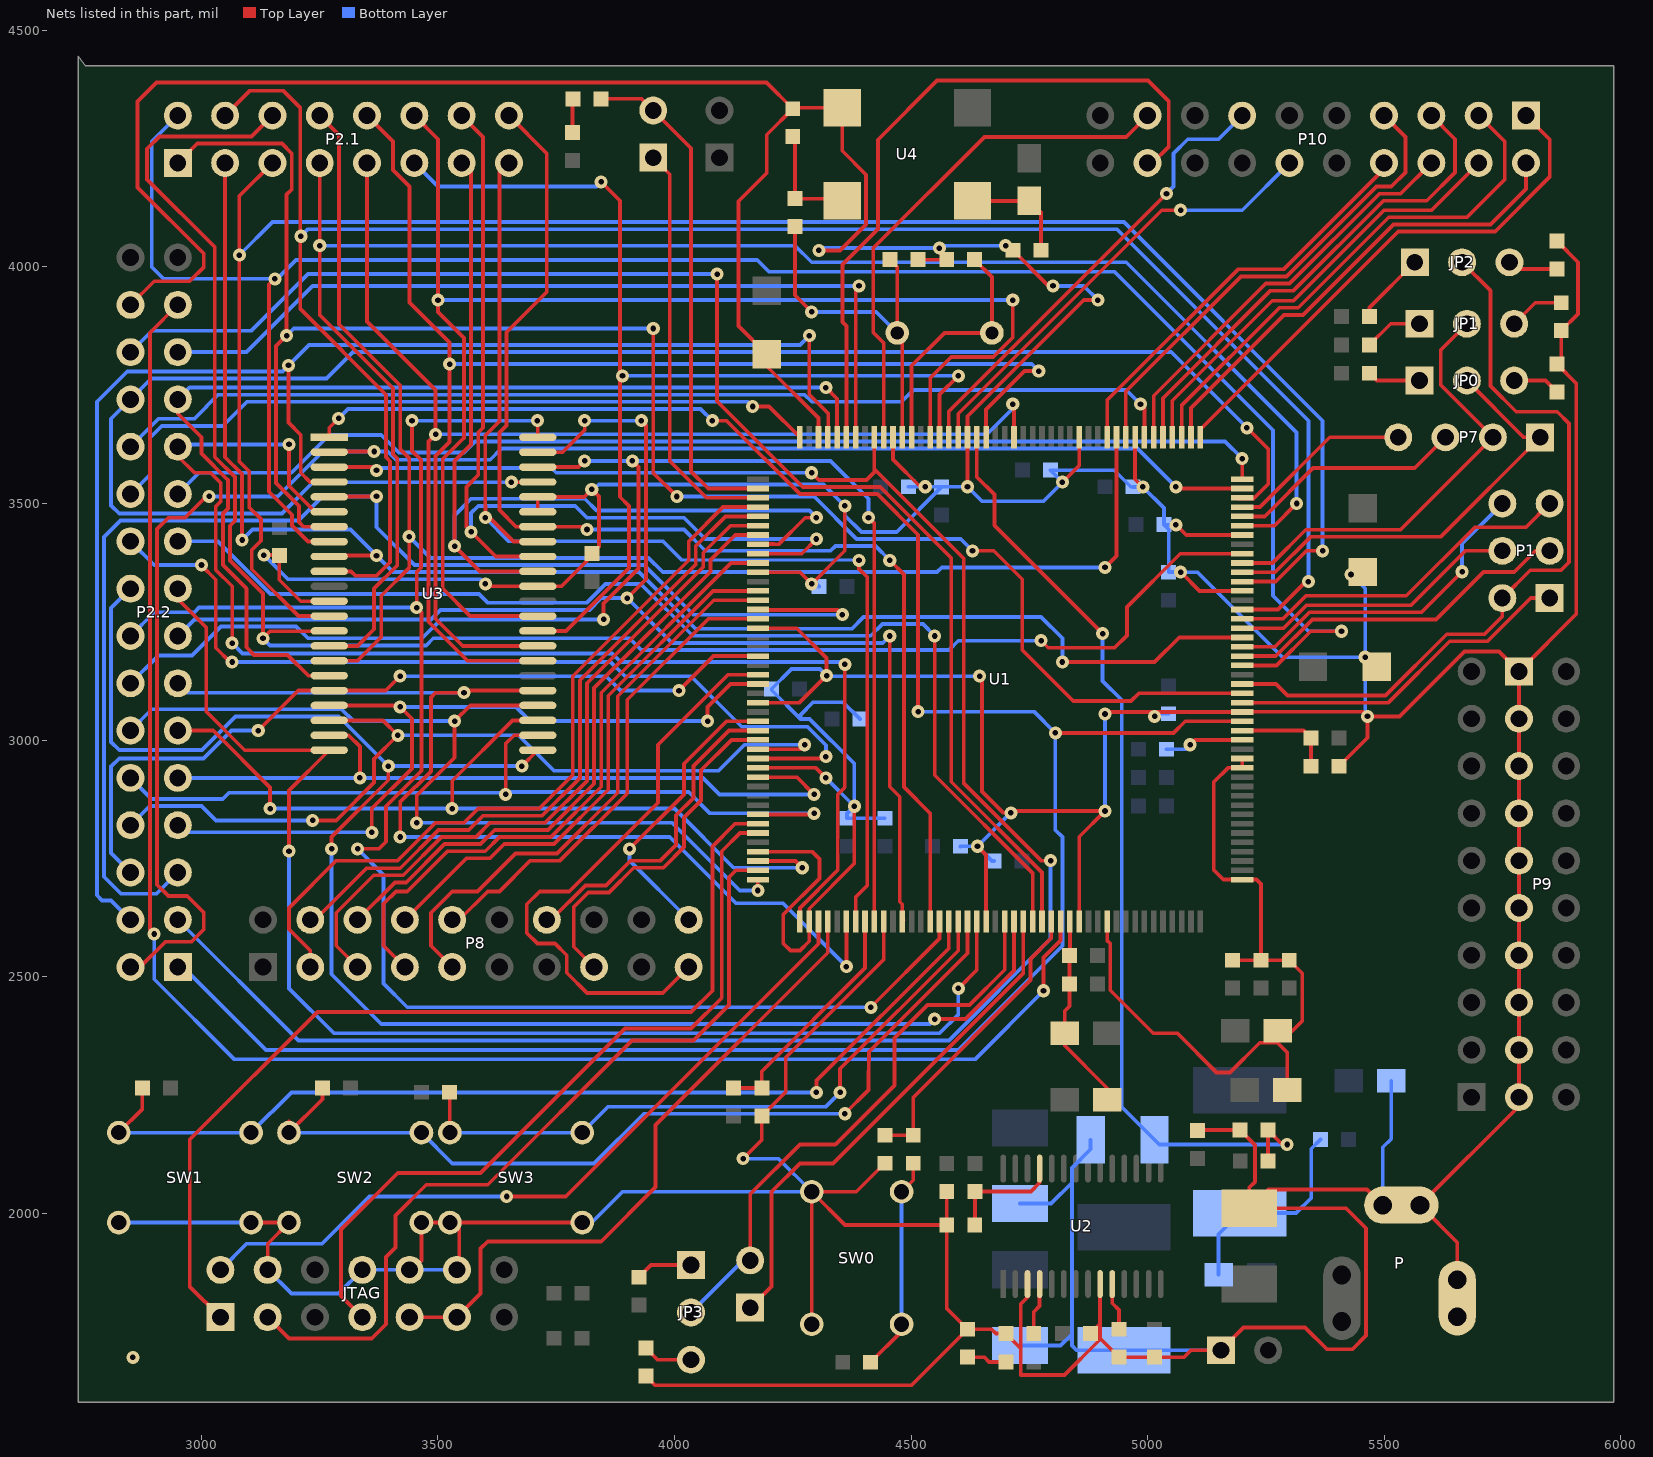
[diagram p0: the nets of this part, all layers, seen from the top]
# Altium PCB MISC76198.PCBDOC (part 2 of 2)
Units mil, origin at the board's own origin, x right, y up, seen from the top; angles counter-clockwise.
Board outline 3245 x 2845 mil, 2 copper layers (Top Layer, Bottom Layer); 107 components, 158 nets, 601 pads, 196 vias.

## Via types
v1: diameter 27.56, hole 11.81, Top Layer to Bottom Layer, 194 vias
v2: diameter 39.37, hole 19.68, Top Layer to Bottom Layer, 2 vias

## Nets (pads, with @x,y where several pads share a name; then routed paths per layer and width w, separated by ;. In a path a pad name is that pad's centre, name@x,y a point inside that pad or via, vN(x,y) a via of type N, cw(c..) or ccw(c..) an arc to the next point about the centre after c; other vN are vias at no path point) (continued)
GND: C1.2 C2.2 C3.2 C4.1 C5.2 C6.1 C7.2 C10.2 C11.2 C12.1 C13.1 C14.1 C15.1 C16.1 C17.2 C25.1 C26.1 C29.2 C30.1 C31.1 C32.1 C33.1 C34.1 C35.1 C36.1 C37.1 C38.1 C39.1 C40.1 C41.2 C42.1 C43.2 C44.2 C45.2 D1.2 JTAG.4 JTAG.8 JTAG.10 JTAG.12 L2.1 P2.2.30 P9.1 P9.3 P9.5 P9.7 P9.9 P9.11 P9.13 P9.15 P9.17 P9.19 P.2 P.2A P.2B P.3 P.3A P.3B POWER.1 R1.1 R2.1 R5.2 R16.1 R18.1 R20.1 R22.1 R24.1 R26.1 SW0.1 SW0.2 SW1.3 SW1.4 SW2.3 SW2.4 SW3.3 SW3.4 U1.19 U1.32 U1.38 U1.52 U1.58 U1.70 U1.78 U1.86 U1.99 U1.105 U1.113 U1.120 U1.129 U1.134 U1.142 U1.153 U1.163 U2.3 U2.9 U3.12 U3.34 U3.39 U3.40 U4.2 | length 25253.5
  Top Layer w8: P2.2.30@2850,3920 2900,3970 2975,3970 3005,4000 3005,4028 2865,4168 2865,4350 2905,4390 4194.61,4390 C14.1@4250,4334.61 ; SW1.3@3105,1980 SW2.4@3185,1980 3140,1935 JTAG.4@3140,1880 ; v1(3132,3391) 3163.95,3391 C26.1@3164.56,3390.39 3164.56,3338.98 3210,3293.54 U3.12@3270,3293.54 ; JTAG.10@3435,1870 3465,1900 SW2.3@3465,1980 SW3.3@3825,1980 ; JTAG.12@3540,1880 3545,1885 SW3.4@3545,1980 ; v1(3600,3330) 3604.96,3325.04 3761.04,3325.04 3825.44,3389.44 C25.1@3825.44,3394.61 3840.22,3409.39 3840.22,3514.78 v1(3825,3530) 3809.02,3514.02 U3.40@3710.94,3514.02 U3.39@3710.94,3482.52 ; R24.1@3939.56,1655.39 3958.95,1636 4501.11,1636 D1.2@4619.56,1754.45 ; v1(4145,2115) 4184.56,2154.56 R26.1@4184.56,2205.39 4235,2255.83 4235,2328.79 4442.13,2535.91 U1.142@4442.13,2616.42 ; U1.129@4176.38,2764.06 4290.94,2764.06 4306.27,2748.73 4306.27,2707.48 4230,2631.21 4230,2570 4245,2555 4265,2555 4284.65,2574.65 4284.65,2643.43 4380,2738.79 v1(4380,2860) ; U1.120@4176.38,2941.22 4298.78,2941.22 v1(4320,2920) ; U1.113@4176.38,3079.02 4264.22,3079.02 v1(4321.43,3136.22) 4321.43,3173.57 4258.5,3236.5 U1.105@4176.38,3236.5 ; U1.99@4176.38,3354.61 4265.39,3354.61 v1(4290,3330) 4360,3400 v1(4360,3495) ; SW0.2@4290,1765 SW0.1@4290,2045 ; U1.86@4304.33,3640.04 4304.33,3680.67 4195,3790 C43.2@4195,3815.17 4135,3875.17 4135,4138.79 4195,4198.79 4195,4279.61 4252.24,4336.85 U4.2@4354.41,4336.85 4354.41,4245.59 4405,4195 4405,4090 4350,4035 v1(4305,4035) ; C15.1@4444.56,2105.39 4384.17,2045 SW0.1@4290,2045 ; U1.78@4461.81,3640.04 4461.81,3593.19 4519.56,3535.44 v1(4530,3535.44) ; C17.2@4514.45,4015.44 C16.1@4575.39,4015.44 ; v1(4560,4040) 4560,4030.83 C16.1@4575.39,4015.44 ; C16.1@4564.95,4005 C16.1@4575.39,4015.44 ; C10.2@4575.44,2045.55 4575.44,2009.11 4575.55,2009 4575.55,1798.46 D1.2@4619.56,1754.45 ; R5.2@4575.55,1974.56 4360.44,1974.56 SW0.1@4290,2045 ; v1(4619.29,3535.44) 4619.29,3684.29 4865,3930 v1(4895,3930) ; v1(4640.44,2775.44) 4658.66,2757.22 U1.153@4658.66,2616.42 ; v1(4645,3135) 4650,3130 4650,2891.21 4695.16,2846.06 v1(4711.06,2846.06) 4715,2850 v1(4910,2850) 4855.51,2795.51 U1.163@4855.51,2616.42 ; C13.1@4709.56,4035.44 C13.1@4715.39,4035.44 4790.83,3960 v1(4800,3960) ; U2.3@4746.18,1850 4746.18,1822.18 4732,1808 4732,1713.83 ; v1(4820,3545) 4855.51,3580.51 U1.58@4855.51,3640.04 ; C3.2@4879.45,1745.44 4899.72,1765.72 ; U2.9@4899.72,1850 4899.72,1765.72 ; v1(4910,3055) 4914.33,3059.33 U1.19@5200,3059.33 ; U1.52@4973.62,3640.04 4973.62,3551.38 v1(4990,3535) ; v1(5015,3050) v1@5015,3059.33 ; v1(5060,3455) 5081.65,3433.35 U1.38@5200,3433.35 ; v1(5070,3355) 5109.76,3315.24 U1.32@5200,3315.24 ; C6.1@5105.44,2174.61 5106.27,2175.44 C12.1@5195.39,2175.44 5227,2143.83 5227,2066 5215,2054 C1.2@5215,2010 ; U1.19@5200,3059.66 5455.67,3059.33 v1(5465,3050) ; R16.1@5404.61,2944.56 5465,3004.95 v1(5465,3050) ; C44.2@5445,3370 5455,3360 C44.2@5455,3355.17 ; v1(5460,3175) C45.2@5494.83,3175 ; P.3@5536.61,2016.85 P.3B@5497.24,2016.85 5464.09,2050 5255,2050 C1.2@5215,2010 ; P.2B@5654.72,1780.63 5654.72,1938.11 P.3A@5575.98,2016.85 5785,2225.87 P9.3@5785,3045 P9.1@5785,3145 ; P.2@5654.72,1820 P.2A@5654.72,1859.37 ; R22.1@5865.44,4054.61 5910,4010.05 5910,3900.83 R20.1@5874.56,3865.39 5874.56,3803.73 R18.1@5865.44,3794.61 5906,3754.05 5906,3266 P9.1@5785,3145 ; D1.2@4619.56,1754.45 4670.39,1754.45 4679.4,1745.44 R1.1@4700.39,1745.44 4732,1713.83 ; 4732,1713.83 4732,1658 4824.72,1658 4895.81,1729.08 4899.72,1733 ; 4899.72,1733 4899.72,1765.72 ; 4899.72,1733 4899.72,1735.23 R2.1@4939.56,1695.39 C4.1@5014.56,1695.39 5077,1695.39 5091.61,1710 POWER.1@5155,1710 5203,1758 5333,1758 5379,1712 5433,1712 5462,1741 5462,1968 5420,2010 C1.2@5215,2010 ; v1(5465,3050) 5532.68,3050 5669.86,3187.17 5742.83,3187.17 P9.1@5785,3145
  Bottom Layer w8: SW1.4@2825,1980 SW1.3@3105,1980 ; v1(3132,3391) 3183,3340 3590,3340 v1(3600,3330) ; JTAG.4@3140,1880 3190,1830 3290,1830 JTAG.8@3340,1880 JTAG.12@3540,1880 ; SW3.3@3825,1980 3890,2045 SW0.1@4290,2045 4220,2115 v1(4145,2115) ; v1(3825,3530) 3840.65,3540 4315,3540 v1(4360,3495) 4360,3475 4395,3440 4469.95,3440 C32.1@4564.56,3534.61 4563.73,3535.44 C40.1@4494.61,3535.44 ; v1(4290,3330) 4299.95,3330 C33.1@4305.39,3324.56 ; v1(4305,4035) 4310,4040 v1(4560,4040) 4565,4045 v1(4700,4045) ; v1(4320,2920) v1(4380,2860) ; v1(4321.43,3136.22) 4307.65,3150 4247.14,3150 C34.1@4205.39,3108.25 4205.39,3105.33 4266.09,3044.63 ; v1@4322.65,3135 v1(4645,3135) ; C41.2@4391.89,3044.56 4356.45,3080 4292.84,3080 4266.09,3053.25 4266.09,3044.63 ; C36.1@4444.56,2834.61 C35.1@4364.56,2834.61 4364.56,2844.56 v1(4380,2860) ; C32.1@4565.39,3535.44 v1@4625,3535.44 ; C42.1@4604.61,2774.34 C42.1@4604.61,2775.44 v1(4640.44,2775.44) ; v1(4619.29,3535.44) 4649.34,3505.39 4780,3505 ; C37.1@4675.39,2744.56 4671.32,2744.56 v1(4640.44,2775.44) ; v1@4710.53,2845.53 v1(4640.44,2775.44) ; C7.2@4730,1720 4816,1720 4840,1744 4840,1720 ; C5.2@4730,2020 4796,2020 4840,2064 ; 4780.39,3505.39 v1(4820,3545) v1(4820,3545) C39.1@4794.61,3570.44 4929.61,3570.44 C31.1@4964.61,3535.44 ; v1(4800,3960) 4865,3960 v1(4895,3930) ; C11.2@4879.65,2154.88 4879.65,2135 4840,2095.35 4840,2064 ; v1@4910,2855 v1(4910,3055) ; C31.1@4969.49,3535 v1(4990,3535) 5034.61,3490.39 C30.1@5034.61,3455.44 5044.56,3445.49 C38.1@5044.56,3354.61 5044.95,3355 v1(5070,3355) 5070.39,3354.61 5105.39,3354.61 5285,3175 v1(5460,3175) ; v1(5015,3050) 5020.55,3055.55 C29.2@5044.56,3055.55 ; C30.1@5035.05,3455 v1(5060,3455) ; POWER.1@5155,1710 C2.2@4950,1710 4850,1710 4840,1720 ; v1(5430,3350) 5460,3320 5460,3055 v1(5465,3050) ; L2.1@5515.15,2279.92 5515.15,2156.91 5497.24,2139 P.3B@5497.24,2016.85 P.3@5536.61,2016.85 P.3A@5575.98,2016.85 ; P.2B@5654.72,1780.63 P.2@5654.72,1820 ; 4266.09,3044.63 4285.62,3044.63 4380,2950.25 v1(4380,2860) ; 4840,1720 4840,2064
  other v1: 2855,1695
MCLKRA: P1.3 U1.25 | length 742.2
  Top Layer w8: U1.25@5200,3177.44 5270.86,3177.44 5348.42,3255 5610.03,3255 5710.03,3355 5775,3355 5820,3400 P1.3@5850,3400
MCLKXA: P1.4 U1.28 | length 617.7
  Top Layer w8: U1.28@5200,3236.5 5287.49,3236.5 5335.99,3285 5556.88,3285 5671.88,3400 P1.4@5750,3400
MDRA: P1.1 U1.20 | length 741.5
  Top Layer w8: U1.20@5200,3079.02 5509.02,3079.02 5638.75,3208.75 5718.75,3208.75 5810,3300 P1.1@5850,3300
MDXA: JP2.2 P1.2 U1.22 | length 1618.7
  Top Layer w8: U1.22@5200,3118.39 5271.61,3118.39 5295.98,3094.02 5502.8,3094.02 5632.53,3223.75 5712.22,3223.75 5750,3261.53 P1.2@5750,3300 5809,3359 5874,3359 5891,3376 5891,3669 5866,3694 5779.47,3694 5725,3748.47 5725,3950 JP2.2@5665,4010
MFSRA: P1.5 U1.29 | length 751
  Top Layer w8: U1.29@5200,3256.18 5285.96,3256.18 5334.78,3305 5546.88,3305 5691.88,3450 5800,3450 P1.5@5850,3500
MFSXA: P1.6 U1.26 | length 710.2
  Top Layer w8: U1.26@5200,3197.13 5269.33,3197.13 5342.21,3270 5579.25,3270 v1(5665,3355.75)
  Bottom Layer w8: v1(5665,3355.75) 5665,3415 P1.6@5750,3500
Net30M_2: 30M.2 C16.2 U1.76 | length 519.4
  Top Layer w8: U1.76@4501.18,3640.04 4501.18,3791.18 4570.75,3860.75 30M.2@4670.87,3860.75 4670.87,3979.02 C16.2@4634.45,4015.44
NetC8_1: C8.1 C9.2 L1.2 | length 444.5
  Bottom Layer w8: L1.2@5150.15,1869.92 5150.15,1955.15 C8.1@5195,2000 5314,2000 5346,2032 5346,2135.89 C9.2@5365.55,2155.44
NetC13_2: C13.2 L3.1 U4.4 | length 234.6
  Top Layer w8: U4.4@4630,4140 4630.3,4139.7 L3.1@4750.16,4139.7 4774.45,4115.41 C13.2@4774.45,4035.44
NetC14_2: C14.2 R9.2 U4.3 | length 234.7
  Top Layer w8: C14.2@4250,4275.55 4254.56,4270.99 R9.2@4254.56,4144.45 4349.96,4144.45 U4.3@4354.41,4140
NetC15_2: C15.2 R8.2 U1.160 | length 632.9
  Top Layer w8: C15.2@4444.56,2164.45 R8.2@4504.56,2164.45 4504.56,2244.56 4752.4,2492.4 4752.4,2537.4 4796.46,2581.46 U1.160@4796.46,2616.42
NetC18_2: C18.2 C19.2 C20.1 L4.2 U1.162 | length 418.3
  Top Layer w8: U1.162@4835.83,2616.42 4835.83,2545.23 C18.2@4835.16,2544.56 4835.16,2437.31 4824.85,2427 C20.1@4824.85,2379.92 4824.85,2354 4914.85,2264 L4.2@4914.85,2239.92
NetD1_1: D1.1 R3.1 | length 85
  Top Layer w8: D1.1@4619.56,1695.39 4655,1695.39 4664.95,1685.44 R3.1@4700.39,1685.44
NetD2_1: D2.1 R100.2 | length 70.2
  Top Layer w8: R100.2@3784.56,4284.45 D2.1@3784.56,4354.61
NetJP0_1: JP0.1 R17.2 | length 111.9
  Top Layer w8: R17.2@5469.45,3775.44 5484.89,3760 JP0.1@5575,3760
NetJP0_3: JP0.3 R18.2 | length 100.6
  Top Layer w8: JP0.3@5775,3760 5840.99,3760 R18.2@5865.44,3735.55
NetJP1_1: JP1.1 R19.2 | length 124
  Top Layer w8: R19.2@5469.45,3835.44 5514.01,3880 JP1.1@5575,3880
NetJP1_3: JP1.3 R20.2 | length 118
  Top Layer w8: JP1.3@5775,3880 5819.45,3924.45 R20.2@5874.56,3924.45
NetJP2_1: JP2.1 R21.2 | length 154.1
  Top Layer w8: R21.2@5469.45,3895.44 5469.45,3914.45 JP2.1@5565,4010
NetJP2_3: JP2.3 R22.2 | length 106.4
  Top Layer w8: JP2.3@5765,4010 5779.45,3995.55 R22.2@5865.44,3995.55
NetJP3_1: JP3.1 R23.2 | length 121
  Top Layer w8: R23.2@3924.56,1864.45 3950.11,1890 JP3.1@4035,1890
NetJP3_3: JP3.3 R24.2 | length 105.6
  Top Layer w8: R24.2@3939.56,1714.45 3964.01,1690 JP3.3@4035,1690
NetR1_2: R1.2 U2.4 | length 109.7
  Top Layer w8: R1.2@4759.45,1745.44 4759.45,1791 4771.77,1803.32 U2.4@4771.77,1850
NetR2_2: R2.2 U2.10 | length 101.5
  Top Layer w8: U2.10@4925.32,1850 4925.32,1809.24 4939.56,1795 R2.2@4939.56,1754.45
NetR4_2: R4.2 R5.1 U2.25 | length 245.4
  Top Layer w8: R5.1@4634.61,1974.56 4635.44,1975.39 R4.2@4635.44,2045.55 4753.32,2045.55 4771.77,2064 U2.25@4771.77,2094.09
NetR7_1: R7.1 R8.1 SW0.3 SW0.4 | length 443
  Top Layer w8: R7.1@4414.61,1684.56 SW0.4@4480,1749.95 ; SW0.3@4480,2045 4504.56,2069.56 R8.1@4504.56,2105.39
  Bottom Layer w8: SW0.4@4480,1765 SW0.3@4480,2045
NetR27_1: R27.1 U1.16 | length 168.6
  Top Layer w8: v1(5090,2990) 5100.28,3000.28 U1.16@5200,3000.28
  Bottom Layer w8: R27.1@5039.61,2980.44 5080.44,2980.44 v1(5090,2990)
PWM1: P8.3 U1.92 | length 1631.8
  Top Layer w8: P8.3@3230,2520 3230,2555 3185,2600 3185,2645 3285,2745 3415,2745 3495,2825 3555,2825 3585,2855 3713.93,2855 3785,2926.07 3785,3135 4030,3380 4030,3420 4102.4,3492.4 U1.92@4176.38,3492.4
PWM2: P8.4 U1.93 | length 1443.2
  Top Layer w8: P8.4@3230,2620 3240,2620 3349.1,2729.1 3420.32,2729.1 3501.21,2810 3565,2810 3595,2840 3720.15,2840 3800,2919.85 3800,3126.21 4045,3371.21 4045,3410 4107.72,3472.72 U1.93@4176.38,3472.72
PWM3: P8.5 U1.94 | length 1502.3
  Top Layer w8: P8.5@3330,2520 3285,2565 3285,2635 3364.1,2714.1 3426.53,2714.1 3507.43,2795 3580,2795 3610,2825 3726.36,2825 3815,2913.64 3815,3120 4060.76,3365.76 4060.76,3395.76 4118.03,3453.03 U1.94@4176.38,3453.03
PWM4: P8.6 U1.95 | length 1316.6
  Top Layer w8: P8.6@3330,2620 3409.1,2699.1 3432.74,2699.1 3513.64,2780 3590,2780 3620,2810 3732.57,2810 3830,2907.43 3830,3110 4075.76,3355.76 4075.76,3380.76 4128.35,3433.35 U1.95@4176.38,3433.35
PWM5: P8.7 U1.98 | length 1358.7
  Top Layer w8: P8.7@3430,2520 3385,2565 3385,2653.79 3411.21,2680 3434.85,2680 3519.85,2765 3600,2765 3630,2795 3738.79,2795 3845,2901.21 3845,3100 4119.29,3374.29 U1.98@4176.38,3374.29
PWM6: P8.8 U1.101 | length 1150.8
  Top Layer w8: P8.8@3430,2620 3560,2750 3610,2750 3640,2780 3745,2780 3860,2895 3860,3093.79 4081.45,3315.24 U1.101@4176.38,3315.24
PWM7: P10.1 U1.45 | length 1126.7
  Top Layer w8: U1.45@5111.42,3640.04 5111.42,3656.42 5530,4075 5735,4075 5850,4190 5850,4270 P10.1@5800,4320
PWM8: P10.2 U1.46 | length 1016.9
  Top Layer w8: U1.46@5091.73,3640.04 5091.73,3701.73 5288.65,3898.65 5328.65,3898.65 5520,4090 5725,4090 5800,4165 P10.2@5800,4220
PWM9: P10.3 U1.47 | length 1105.7
  Top Layer w8: U1.47@5072.05,3640.04 5072.05,3707.05 5278.65,3913.65 5318.65,3913.65 5510,4105 5675,4105 5755,4185 5755,4265 P10.3@5700,4320
PWM10: P10.4 U1.48 | length 933.2
  Top Layer w8: U1.48@5052.36,3640.04 5052.36,3717.36 5263.65,3928.65 5308.65,3928.65 5500,4120 5600,4120 P10.4@5700,4220
PWM11: P10.5 U1.49 | length 1038.4
  Top Layer w8: U1.49@5032.68,3640.04 5032.68,3722.68 5260,3950 5308.79,3950 5498.79,4140 5590,4140 5650,4200 5650,4270 P10.5@5600,4320
PWM12: P10.6 U1.50 | length 878.8
  Top Layer w8: U1.50@5012.99,3640.04 5012.99,3727.99 5250,3965 5300,3965 5490,4155 5535,4155 P10.6@5600,4220
SCIRXDA: P3.1 U1.157 | length 1096.6
  Top Layer w8: P3.1@4160,1800 4205,1845 4205,2045 4265,2105 4335,2105 4737.4,2507.4 U1.157@4737.4,2616.42
SCIRXDB: P6.1 U1.91 | length 874.1
  Top Layer w8: P6.1@3955,4231 3990,4196 3990,3590 4067.91,3512.09 U1.91@4176.38,3512.09
SCITXDA: JP3.2 P3.2 U1.155 | length 1205.8
  Top Layer w8: P3.2@4160,1900 4160,2040 4265,2145 4340,2145 4465,2270 4465,2370 4535,2440 4623.79,2440 4698.03,2514.25 U1.155@4698.03,2616.42
  Bottom Layer w8: JP3.2@4035,1790 4145,1900 P3.2@4160,1900
SCITXDB: D2.2 P6.2 U1.90 | length 1073.2
  Top Layer w8: D2.2@3844.45,4355.44 3930.56,4355.44 4035,4251 4035,3568 4071.23,3531.77 U1.90@4176.38,3531.77
SPICLKA: JP0.2 P7.1 U1.34 | length 952.9
  Top Layer w8: U1.34@5200,3354.61 5269.61,3354.61 5344.55,3429.55 5619.55,3429.55 P7.1@5830,3640 5795,3640 JP0.2@5675,3760
SPIMIMOA: P7.3 U1.40 | length 499.3
  Top Layer w8: U1.40@5200,3472.72 5247.72,3472.72 5350,3575 5565,3575 P7.3@5630,3640
SPIMOMIA: P7.4 U1.41 | length 391.1
  Top Layer w8: U1.41@5200,3492.4 5237.4,3492.4 5385,3640 P7.4@5530,3640
SPISETA: JP1.2 P7.2 U1.35 | length 948.4
  Top Layer w8: U1.35@5200,3374.29 5264.29,3374.29 5334.55,3444.55 5534.55,3444.55 P7.2@5730,3640 5620,3750 5620,3825 JP1.2@5675,3880
T1CTRIP-PDPINTA: P8.19 U1.110 | length 1261.4
  Top Layer w8: P8.19@4030,2520 3975,2465 3815,2465 3772.02,2507.98 3772.02,2545 3747.02,2570 3710,2570 3687.77,2592.23 3687.77,2652.77 3715,2680 3777.57,2680 3965,2867.43 3965,2990 4113.07,3138.07 U1.110@4176.38,3138.07
T1PWM-T1CMP: P8.9 U1.102 | length 1218.2
  Top Layer w8: P8.9@3530,2520 3485,2565 3485,2635 3530,2680 3583.79,2680 3663.79,2760 3751.51,2760 3880,2888.49 3880,3092.57 4082.98,3295.55 U1.102@4176.38,3295.55
T2CTRIP-EVASOC: P8.20 U1.115 | length 622.9
  Top Layer w8: v1(3905,2770) 4020,2885 4020,2950 4109.65,3039.65 U1.115@4176.38,3039.65
  Bottom Layer w8: v1(3905,2770) 3905,2745 P8.20@4030,2620
T2PWM-T2CMP: P8.10 U1.104 | length 1025.7
  Top Layer w8: P8.10@3530,2620 3545,2620 3605,2680 3630.15,2680 3695.15,2745 3757.72,2745 3900,2887.28 3900,3085 4071.18,3256.18 U1.104@4176.38,3256.18
T3CTRIP-PDPINTB: P10.17 U1.79 | length 1105.1
  Top Layer w8: U1.79@4442.13,3640.04 4442.13,3839.07 4420,3861.19 4420,4040 4655,4275 4955,4275 P10.17@5000,4320
T3PWM-T3CMP: P10.7 U1.53 | length 1018.2
  Top Layer w8: U1.53@4953.94,3640.04 4953.94,3736.51 5197.43,3980 5293.79,3980 5483.79,4170 5515,4170 5545,4200 5545,4275 P10.7@5500,4320
T4CTRIP-EVBSOC: P10.18 U1.83 | length 1503
  Top Layer w8: U1.83@4363.39,3640.04 4363.39,3875.38 4355,3883.77 4355,4005 4430,4080 4430,4269 4555,4394 5001,4394 5045,4350 5045,4255 5010,4220 P10.18@5000,4220
T4PWM-T4CMP: P10.8 U1.55 | length 918.9
  Top Layer w8: U1.55@4914.57,3640.04 4914.57,3718.35 5191.21,3995 5287.57,3995 P10.8@5500,4207.43 ; P10.8@5490,4197.43 P10.8@5490,4240 ; P10.8@5500,4210 P10.8@5500,4220
TCK: JTAG.9 JTAG.11 U1.136 | length 1401.8
  Top Layer w8: JTAG.9@3440,1780 JTAG.11@3540,1780 3590,1830 3590,1925 3605,1940 3845,1940 3960,2055 3960,2186.21 4324.02,2550.23 U1.136@4324.02,2616.42
TCLINB: P10.13 U1.72 | length 974.9
  Top Layer w8: U1.72@4579.92,3640.04 4579.92,3694.92 v1(5040,4155)
  Bottom Layer w8: v1(5040,4155) 5055,4170 5055,4240 5085,4270 5150,4270 P10.13@5200,4320
TCLKINA: P8.15 U1.117 | length 763.1
  Top Layer w8: P8.15@3830,2520 3787.02,2562.98 3787.02,2647.02 3817.78,2677.78 3861.56,2677.78 3913.79,2730 3976.36,2730 4020,2773.64 4020,2836.21 4056.02,2872.23 4056.02,2936.02 4120.28,3000.28 U1.117@4176.38,3000.28 ; U1.117@4176.38,3000 U1.117@4185,3000
TDI: JTAG.3 U1.131 | length 1746.1
  Top Layer w8: JTAG.3@3140,1780 3185,1735 3360,1735 3390,1765 3390,1907.25 3410,1927.25 3410,1995 3475,2060 3605,2060 3910,2365 4040,2365 4115,2440 4115,2710 4129.69,2724.69 U1.131@4176.38,2724.69
TDIRA: P8.14 U1.116 | length 688.3
  Top Layer w8: P8.14@3730,2620 3738.79,2620 3811.56,2692.78 3855.35,2692.78 3907.57,2745 3970.15,2745 4003.4,2778.25 4003.4,2840.83 4040,2877.43 4040,2945 4114.96,3019.96 U1.116@4176.38,3019.96
TDIRB: P10.12 U1.71 | length 1009.7
  Top Layer w8: U1.71@4599.61,3640.04 4599.61,3689.61 5030,4120 v1(5070,4120) ; P10.12@5300,4220 5290,4220 5290,4240 P10.12@5300,4240
  Bottom Layer w8: v1(5070,4120) 5200,4120 P10.12@5300,4220
TDO: JTAG.7 U1.127 | length 1613.9
  Top Layer w8: JTAG.7@3340,1780 3295,1825 3295,1965 3415,2085 3590,2085 3895,2390 4035,2390 4100,2455 4100,2765 4138.43,2803.43 U1.127@4176.38,2803.43
TMS: JTAG.1 U1.126 | length 2058.7
  Top Layer w8: JTAG.1@3040,1780 2975,1845 2975,2155 3245,2425 4035,2425 4080,2470 4080,2775 4128.11,2823.11 U1.126@4176.38,2823.11
TRST: JTAG.2 U1.135 | length 1596.9
  Top Layer w8: v1(3645,2035) 3770,2035 4304.33,2569.33 U1.135@4304.33,2616.42
  Bottom Layer w8: JTAG.2@3040,1880 3095,1935 3255,1935 3355,2035 v1(3645,2035)
VDD3VFL: C11.1 C12.2 R6.1 U1.69 | length 2044
  Top Layer w8: U1.69@4638.98,3640.04 4638.98,3556.02 4676.14,3518.86 4676.14,3453.86 v1(4905,3225) ; R6.1@5255,2110 5254.45,2110.55 C12.2@5254.45,2175.44 5284.89,2145 v1(5295,2145)
  Bottom Layer w8: v1(4905,3225) 4905,3125 4945.42,3084.58 4945.42,2224.11 5024.54,2145 v1(5295,2145)
VDDA1: C21.2 C22.2 C23.2 C24.1 L5.1 U1.1 U1.13 U1.14 U1.166 | length 1605.5
  Top Layer w8: U1.166@4914.57,2616.42 4914.57,2576.43 4921,2570 4921,2471 5012,2380 5063,2380 5146,2297 5174,2297 5237,2360 5274.93,2360 5275.15,2359.78 ; C21.2@5179.56,2534.45 C22.2@5239.56,2534.45 ; U1.14@5200,2960.91 U1.13@5200,2941.22 5170,2941.22 5140,2911.22 5140,2725 5160,2705 5230.56,2705 5239.56,2696 C22.2@5239.56,2534.45 ; L5.1@5295.15,2260.08 5295.15,2339.78 5275.15,2359.78 ; C22.2@5239.56,2534.45 C23.2@5299.56,2534.45 5327,2507.01 5327,2406.08 5306,2385.08 C24.1@5275.15,2385.08 5275.15,2359.78
X1: 30M.1 C17.1 R9.1 U1.77 | length 780.5
  Top Layer w8: R9.1@4254.56,4085.39 4254.56,3940.44 v1(4290,3905) ; C17.1@4455.39,4015.44 4470.87,3999.96 30M.1@4470.87,3860.75 4481.5,3850.12 U1.77@4481.5,3640.04
  Bottom Layer w8: v1(4290,3905) 4426.61,3905 30M.1@4470.87,3860.75
XA0: P2.2.1 U1.18 U3.1 | length 4958.1
  Top Layer w8: U3.1@3270,3640 3270,3660 v1(3290,3680) ; v1(4080,3675) 4110,3675 4265,3520 4428.79,3520 4515,3433.79 v1(4515,3060) ; v1(4805,3015) 5055,3015 5079.65,3039.65 U1.18@5200,3039.65
  Bottom Layer w8: P2.2.1@2961.21,2520 3136.21,2345 4600,2345 4820,2565 4820,2795 4805,2810 v1(4805,3015) 4760,3060 v1(4515,3060) ; v1(3290,3680) 3310,3700 4055,3700 v1(4080,3675)
XA1: P2.2.2 U1.43 U3.2 | length 3608.3
  Top Layer w8: P2.2.2@2850,2520 2870,2520 2923.36,2573.36 2978.36,2573.36 3005,2600 3005,2635 2970,2670 2930,2670 2906,2694 2906,3446 2930,3470 2965,3470 3010,3515 v1(3016,3515) ; U3.2@3270,3608.5 3271.5,3610 v1(3365,3610) ; v1(5060,3535) 5063.23,3531.77 U1.43@5200,3531.77
  Bottom Layer w8: v1(3016,3515) 3161.21,3515 3256.21,3610 3393.79,3610 3411.41,3592.38 3610.38,3592.38 3634.22,3616.22 4978.78,3616.22 v1(5060,3535)
XA2: P2.2.3 U1.80 U3.3 | length 4451.3
  Top Layer w8: U3.3@3270,3577.01 3362.99,3577.01 v1(3370,3570) ; v1(4290,3565) 4305,3550 4405.78,3550 4422.44,3566.66 U1.80@4422.44,3640.04 ; 4422.44,3572.56 4611.63,3383.37 4611.63,2908.37 4775,2745 v1(4795,2745)
  Bottom Layer w8: P2.2.3@2955,2620 P2.2.3@2950,2620 3205,2365 4580,2365 4795,2580 v1(4795,2745) ; v1(3370,3570) 3375,3575 3740,3575 3750,3565 v1(4290,3565)
XA3: P2.2.4 U1.85 U3.4 | length 3237.3
  Top Layer w8: v1(3184,3792) 3184,3671 3210,3645 3210,3565 3229.49,3545.51 U3.4@3270,3545.51 ; v1(4285,3855) 4285,3730 4325,3690 4325,3641.02 U1.85@4324.02,3640.04
  Bottom Layer w8: P2.2.4@2850,2620 2809,2661 2790,2661 2779,2672 2779,3715 2843,3779 3171,3779 3227,3835 4265,3835 v1(4285,3855)
XA4: P2.2.5 U1.103 U3.5 | length 2930
  Top Layer w8: U3.5@3270,3514.02 3270.98,3515 v1(3370,3515) ; U1.103@4175.51,3275 U1.103@4176.38,3275.87 ; U1.103@4176.38,3275 4345,3275 v1(4355,3265)
  Bottom Layer w8: P2.2.5@2949.79,2720 2904.79,2675 2830,2675 2794,2711 2794,3429 2829,3464 3205,3464 3256,3515 v1(3370,3515) 3370,3450 3450,3370 3935.32,3370 4040.32,3265 v1(4355,3265)
XA5: P2.2.6 U1.108 U3.18 | length 1730.3
  Top Layer w8: v1(3120,3020) 3204.57,3104.57 3389.57,3104.57 v1(3420,3135) ; v1(4009.53,3104.53) 4082.44,3177.44 U1.108@4176.38,3177.44
  Bottom Layer w8: P2.2.6@2850,2720 2809,2761 2809,2944 2826,2961 3004.21,2961 3063.21,3020 v1(3120,3020) ; v1(3420,3135) 3855,3135 3885.47,3104.53 v1(4009.53,3104.53)
XA6: P2.2.7 U1.111 U3.19 | length 1706
  Top Layer w8: U3.19@3270,3073.07 3416.93,3073.07 3445,3045 3445,2940 3360,2855 v1(3360,2805) ; v1(4070,3040) 4070,3070 4118.39,3118.39 U1.111@4176.38,3118.39
  Bottom Layer w8: P2.2.7@2945,2830 2970,2805 v1(3360,2805) ; v1(3420,3070) 3665,3070 3695,3040 v1(4070,3040)
XA7: P2.2.8 U1.118 U3.20 | length 1872.7
  Top Layer w8: v1(3235,2830) 3285,2830 3365,2910 3365,2960 v1(3415,3010) 3383.43,3041.57 U3.20@3270,3041.57 ; U1.118@4176.38,2980.59 4265.59,2980.59 v1(4275,2990)
  Bottom Layer w8: P2.2.8@2850,2820 2890.53,2860.53 3000,2860.53 3030.53,2830 v1(3235,2830) ; v1(3415,3010) 3670,3010 3745,2935 4093.2,2935 4148.2,2990 v1(4275,2990)
XA8: P2.2.9 U1.121 U3.21 | length 1636.4
  Top Layer w8: U3.21@3270,3010.08 3310.92,3010.08 3335,2986 v1(3335,2920) ; U1.121@4177.91,2920 U1.121@4176.38,2921.54 4258.46,2921.54 v1(4295,2885)
  Bottom Layer w8: P2.2.9@2950,2920 4060,2920 4095,2885 v1(4295,2885)
XA9: P2.2.10 U1.125 U3.24 | length 1793
  Top Layer w8: v1(3643,2885) 3643,2992 3661.08,3010.08 U3.24@3710.94,3010.08 ; U1.125@4176.38,2842.8 4292.8,2842.8 v1(4295,2845)
  Bottom Layer w8: P2.2.10@2850,2920 2894.47,2875.53 3045,2875.53 3058.05,2888.58 3639.42,2888.58 v1(3643,2885) 3648,2890 4030,2890 4075,2845 v1(4295,2845)
XA10: P2.2.11 U1.130 U3.25 | length 1858.8
  Top Layer w8: P2.2.11@2950,3020 3025,3020 3145,2900 v1(3145,2855) ; v1(3530,2855) 3530,2914 3657.57,3041.57 U3.25@3710.94,3041.57 ; U1.130@4176.38,2744.37 4255.63,2744.37 v1(4270,2730)
  Bottom Layer w8: v1(3145,2855) 4000,2855 4125,2730 v1(4270,2730)
XA11: P2.2.12 U1.132 U3.26 | length 1955.4
  Top Layer w8: v1(3455,2825) 3455,2882.57 3535,2962.57 v1(3535,3040) 3568.07,3073.07 U3.26@3710.94,3073.07 ; v1(4176,2682) 4176,2705 U1.132@4176.38,2705
  Bottom Layer w8: P2.2.12@2850,3020 2895,3065 3296.21,3065 3321.21,3040 v1(3535,3040) ; v1(3455,2825) 3995,2825 4138,2682 v1(4176,2682)
XA12: P2.2.13 U1.138 U3.27 | length 2319.5
  Top Layer w8: v1(3420,2795) 3420,2868.79 3485,2933.79 3485,3090 3495,3100 v1(3555,3100) 3559.57,3104.57 U3.27@3710.94,3104.57 ; v1(4363.39,2521) U1.138@4363.39,2616.42
  Bottom Layer w8: P2.2.13@2950,3120 2970,3100 v1(3555,3100) ; v1(3420,2795) 3990,2795 4130,2655 4229.39,2655 v1(4363.39,2521)
XA13: P2.2.14 U1.141 U3.42 | length 3084
  Top Layer w8: U3.42@3710.94,3577.01 3797.01,3577.01 v1(3810,3590) ; v1(3850,3255) 3850,3288.57 3924,3362.57 3924,3577 v1(3911,3590) ; v1(4410,3470) 4422.44,3457.56 U1.141@4422.44,2616.42
  Bottom Layer w8: P2.2.14@2850,3120 2909,3179 2980,3179 3041,3240 3200,3240 3225,3215 3466.21,3215 3506.21,3255 v1(3850,3255) ; v1(3810,3590) 4330,3590 4410,3510 v1(4410,3470)
XA14: P2.2.15 U1.144 U3.43 | length 2871
  Top Layer w8: U3.43@3710.94,3608.5 3763.5,3608.5 3810,3655 v1(3810,3675) ; v1(3900,3300) 3940,3340 3940,3665 v1(3930,3675) ; v1(4455,3220) 4455,2901.22 4476.22,2880 4476.22,2658.22 4481.5,2652.94 4481.5,2619.2 4484.28,2619.2 U1.144@4481.5,2616.42
  Bottom Layer w8: P2.2.15@2965,3220 P2.2.15@2950,3220 2985,3255 3485,3255 3505,3275 3820,3275 3845,3300 v1(3900,3300) 3994.68,3205.32 4440.32,3205.32 v1(4455,3220) ; v1(3810,3675) v1(3930,3675)
XA15: P2.2.16 U1.148 U3.44 | length 3533.2
  Top Layer w8: v1(3330,2770) 3375,2770 3390,2785 3390,2860 3465,2935 3465,3270 v1(3455,3280) 3455,3355.35 3463.78,3364.13 3463.78,3592.43 3445,3611.21 v1(3445,3675) ; v1(3710,3675) 3710.94,3674.06 U3.44@3710.94,3640 ; v1(4415,2435) 4560.24,2580.24 U1.148@4560.24,2616.42
  Bottom Layer w8: P2.2.16@2850,3220 2900,3270 2985,3270 2995,3280 v1(3455,3280) ; v1(3330,2770) 3385,2715 3385,2485 3435,2435 v1(4415,2435) ; v1(3445,3675) v1(3710,3675)
XA16: P2.2.17 U1.152 U3.22 | length 2800.8
  Top Layer w8: P2.2.17@2950,3320 2950,3298 3010,3238 3010,3060 3091.42,2978.58 U3.22@3270,2978.58 3185,2893.58 v1(3185,2765) ; v1(4600,2475) 4638.98,2513.98 U1.152@4638.98,2616.42
  Bottom Layer w8: v1(3185,2765) 3185,2475 3280,2380 4560,2380 4600,2420 v1(4600,2475)
XA17: P2.2.18 U1.156 U3.23 | length 3462.9
  Top Layer w8: v1(3275,2770) 3275,2795 3395,2915 v1(3395,2945) ; v1(3677.36,2945) U3.23@3710.94,2978.58 ; v1(4550,2410) 4615,2410 4717.72,2512.72 U1.156@4717.72,2616.42
  Bottom Layer w8: P2.2.18@2850,3320 2809,3279 2809,2996 2826,2979 3001,2979 3071.78,3049.78 3290.22,3049.78 v1(3395,2945) v1(3677.36,2945) ; v1(3275,2770) 3275,2505 3380,2400 4540,2400 v1(4550,2410)
XA18: P2.2.19 U1.158 | length 2425.8
  Top Layer w8: v1(4550,3220) 4550,2925.72 4757.09,2718.63 U1.158@4757.09,2616.42
  Bottom Layer w8: P2.2.19@2950,3420 3035,3420 3146,3309 3586.85,3309 3605.85,3290 3813.79,3290 3853.79,3330 3928.79,3330 4038.47,3220.32 4415,3220.32 4439.68,3245 4525,3245 v1(4550,3220)
XCLKOUT: P2.2.20 U1.119 | length 1901.6
  Top Layer w8: v1@3000,3368.79 3030,3338.79 3030,3195 3060,3165 v1(3065,3165) ; U1.119@4176.38,2960.91 4315.91,2960.91 v1(4320,2965)
  Bottom Layer w8: P2.2.20@2850,3420 2900,3370 v1(3000,3370) ; v1(3065,3165) 3865,3165 3895,3135 4035,3135 4142.05,3027.95 4281.09,3027.95 4320,2989.04 v1(4320,2965)
XD0: P2.1.1 U1.21 U3.7 | length 3780.6
  Top Layer w8: P2.1.1@2950,4220 2991,4261 3170,4261 3191,4240 3191,4164 3180,4153 v1(3180,3855) 3157.78,3832.78 3157.78,3543.43 3206.31,3494.91 3206.31,3460.69 3215.98,3451.02 U3.7@3270,3451.02 ; v1(3955,3870) 3955,3564.79 v1(4005,3514.79) ; v1@4625,3395 v1(4630,3400) 4675,3400 4735,3340 4735,3190 4842.78,3082.22 4965,3082.22 4981.48,3098.7 U1.21@5200,3098.7
  Bottom Layer w8: v1(3180,3855) 3195,3870 v1(3955,3870) ; v1(4005,3514.79) 4295.21,3514.79 4385,3425 4605,3425 v1(4630,3400)
XD1: P2.1.2 U1.24 U3.8 | length 4292.7
  Top Layer w8: v1(3155,3975) 3142.78,3962.78 3142.78,3524.72 3191.31,3476.2 3191.31,3453.69 3225.47,3419.53 U3.8@3270,3419.53 ; U1.24@5200,3157.76 5272.76,3157.76 5345,3230 v1(5410,3230)
  Bottom Layer w8: P2.1.2@2950,4320 2895,4265 2895,4000 2920,3975 v1(3155,3975) ; v1@3157.5,3972.5 3200,4015 4175,4015 4200,3990 4930,3990 5265,3655 5265,3305 5340,3230 v1(5410,3230)
XD2: P2.1.3 U1.27 U3.9 | length 3223.5
  Top Layer w8: P2.1.3@3050,4220 3050,3597.87 3085.78,3562.09 v1(3085.78,3422.78) ; U3.9@3270,3388.03 3271.97,3390 v1(3370,3390) ; v1(4820,3165) 5015,3165 5066.81,3216.81 U1.27@5200,3216.81
  Bottom Layer w8: v1(3085.78,3422.78) 3108,3445 3315,3445 3405,3355 3925,3355 4044.68,3235.32 4375,3235.32 4399.68,3260 4775,3260 4820,3215 v1(4820,3165)
XD3: P2.1.4 U1.30 U3.10 | length 4187.7
  Top Layer w8: P2.1.4@3050,4320 3102.76,4372.76 3172.24,4372.76 3209,4336 3209,3911 3390,3730 3390,3598.03 3398.78,3589.25 3398.78,3376 3370.03,3347.25 3325.5,3347.25 3316.22,3356.54 U3.10@3270,3356.54 ; U1.30@5200,3275.87 5275.87,3275.87 5335,3335 v1(5340,3335)
  Bottom Layer w8: v1(3210,4065) 3225,4080 4935,4080 5340,3675 v1(5340,3335)
XD4: P2.1.5 U1.33 U3.13 | length 4084.8
  Top Layer w8: P2.1.5@3150,4220 3080,4150 3080,3589.08 3100.78,3568.3 3100.78,3492.22 3125.78,3467.22 3125.78,3421.22 3106.22,3401.66 3106.22,3361 3205.17,3262.05 U3.13@3270,3262.05 ; U1.33@5200,3334.92 5271.14,3334.92 5336.21,3400 v1(5370,3400)
  Bottom Layer w8: v1(3080,4025) 3150,4095 4950,4095 5370,3675 v1(5370,3400)
XD5: P2.1.6 U1.36 U3.14 | length 3810
  Top Layer w8: P2.1.6@3150,4320 3106,4276 2911,4276 2885,4250 2885,4185 3028,4042 3028,3598.66 3070.78,3555.88 3070.78,3463.56 3060.22,3453 3060.22,3379.78 3130,3310 v1(3130,3215) 3145,3230 U3.14@3270,3230 ; v1(4775,3210) 4790,3195 4930,3195 4956.27,3221.27 4956.27,3281.27 5068.98,3393.98 U1.36@5200,3393.98
  Bottom Layer w8: v1(3130,3215) 3145,3200 3475,3200 3490,3215 3905,3215 3929.68,3190.32 4580,3190.32 4599.68,3210 v1(4775,3210)
XD6: P2.1.7 U1.39 U3.15 | length 3696.6
  Top Layer w8: P2.1.7@3250,4220 3250,3898.79 3405,3743.79 3405,3604.25 3413.78,3595.47 3413.78,3368.78 3365,3320 3365,3234.05 3330,3199.05 U3.15@3270,3199.05 ; U1.39@5200,3453.03 5268.03,3453.03 v1(5315,3500)
  Bottom Layer w8: v1(3250,4045) 4255,4045 4290,4010 4955,4010 5315,3650 v1(5315,3500)
XD7: P2.1.8 U1.54 U3.16 | length 3127.2
  Top Layer w8: P2.1.8@3250,4320 3291,4279 3291,3879 3420,3750 3420,3615 3439,3596 3439,3364 3380,3305 3380,3217.56 3330,3167.56 U3.16@3270,3167.56 ; v1(4910,3365) 4934.25,3389.25 U1.54@4934.25,3640.04
  Bottom Layer w8: v1(3439,3430) 3484,3385 3945,3385 3975,3355 4555,3355 4565,3365 v1(4910,3365)
XD8: P2.1.9 U1.65 U3.29 | length 2624.1
  Top Layer w8: P2.1.9@3350,4220 3350,3885 3495,3740 v1(3495,3646.22) 3480,3631.22 3480,3250 3562.44,3167.56 U3.29@3710.94,3167.56 ; v1(4715,3710) 4717.72,3707.28 U1.65@4717.72,3640.04
  Bottom Layer w8: v1(3495,3646.22) 4660.22,3646.22 4715,3701 v1(4715,3710)
XD9: P2.1.10 U1.68 U3.30 | length 2842.9
  Top Layer w8: P2.1.10@3350,4320 3405,4265 3405,4205 3440,4170 3440,3925 3524.6,3840.4 3524.6,3630 3495,3600.4 3495,3256.21 3552.16,3199.05 U3.30@3710.94,3199.05 ; U1.68@4658.66,3640.04 4658.66,3698.66 4740,3780 v1(4770,3780)
  Bottom Layer w8: v1@3525,3795 4755,3795 v1(4770,3780)
  other v1: 3524.6,3794.6
XD10: P2.1.11 U1.73 U3.31 | length 2375.7
  Top Layer w8: U3.31@3710.94,3230.55 3770.77,3230.55 3903.78,3363.56 3903.78,3494.78 3884.19,3514.37 3885,3515.18 3885,4140 v1(3845,4180) ; U1.73@4560.24,3640.04 4560.24,3730.24 v1(4600,3770)
  Bottom Layer w8: P2.1.11@3450,4220 3500,4170 3835,4170 v1(3845,4180) ; v1@3880,3770 v1(4600,3770)
  other v1: 3890,3770
XD11: P2.1.12 U1.74 U3.32 | length 2926.7
  Top Layer w8: P2.1.12@3450,4320 3500,4270 3500,3905 3555,3850 3555,3638.79 ; 3555,3639.19 3510,3594.19 3510,3320 3567.95,3262.05 U3.32@3710.94,3262.05 ; U1.74@4540.55,3640.04 4540.55,3765.55 4585,3810 4673.79,3810 4715,3851.21 v1@4715,3940
  Bottom Layer w8: v1(3500,3930) v1(4715,3930)
XD12: P2.1.13 U1.96 U3.35 | length 2079.9
  Top Layer w8: P2.1.13@3550,4220 3570,4200 3570,3625 3535,3590 v1(3535,3410) 3588.46,3356.54 U3.35@3710.94,3356.54 ; U1.96@4170,3415 4211,3415 ; U1.96@4176.38,3413.66 4220,3413.66 4276.34,3470 v1(4300,3470)
  Bottom Layer w8: v1(3535,3410) 3535,3475 3570,3510 3810.37,3510 3835.37,3485 4285,3485 v1(4300,3470)
XD13: P2.1.14 U1.97 U3.36 | length 2021.4
  Top Layer w8: P2.1.14@3550,4320 3595,4275 3595,3660 3585,3650 3585,3560 3560,3535 3560,3450 3621.97,3388.03 U3.36@3710.94,3388.03 ; U1.97@4176.38,3393.98 4268.98,3393.98 v1(4300,3425)
  Bottom Layer w8: v1(3570,3440) 3570,3480 3585,3495 3790,3495 3815,3470 4020,3470 4065,3425 v1(4300,3425)
XD14: P2.1.15 U1.139 U3.37 | length 2505
  Top Layer w8: 3600,3495 3600,3643.79 3630,3673.79 3630,4200 P2.1.15@3650,4220 ; 3600.22,3495 3600.22,3478.78 3659.47,3419.53 U3.37@3710.94,3419.53 ; U1.139@4383.07,2616.42 4383.07,2668.07 4407.44,2692.44 4407.44,3344.41 4390,3361.85 v1(4390,3380)
  Bottom Layer w8: v1(3600,3470) 3650,3420 3976.21,3420 4015.29,3380.92 v1(4390,3380)
XD15: P2.1.16 U1.147 U3.38 | length 2586.2
  Top Layer w8: P2.1.16@3650,4320 3730,4240 3730,3947 3645,3862 3645,3665 3630,3650 3630,3486.02 3665,3451.02 3808.98,3451.02 v1(3815,3445) ; U3.38@3710.94,3451.02 U3.38@3711.97,3450 ; v1(4455,3380) 4485,3350 4485,2900.55 4540.55,2845 U1.147@4540.55,2616.42
  Bottom Layer w8: v1(3815,3445) 4020,3445 4065,3400 4330,3400 4340,3410 4425,3410 v1(4455,3380)
XF-XPLL: R25.2 R26.2 U1.140 | length 509.6
  Top Layer w8: R25.2@4124.56,2264.45 4185.55,2264.45 R26.2@4190,2260 ; R26.2@4184.56,2264.45 4184.56,2299.56 4402.76,2517.76 U1.140@4402.76,2616.42
XHOLDAN: P2.2.27 U1.82 | length 1820.8
  Top Layer w8: U1.82@4383.07,3640.04 4383.07,3953.07 v1(4390,3960)
  Bottom Layer w8: P2.2.27@2950,3820 3095,3820 3235,3960 v1(4390,3960)
XHOLDN: P2.2.28 U1.159 | length 3057.3
  Top Layer w8: v1(4090,3985) 4090,3716.21 4271.21,3535 4435,3535 4585,3385 4585,2911.93 4776.77,2720.16 U1.159@4776.77,2616.42
  Bottom Layer w8: P2.2.28@2850,3820 2895,3865 3105,3865 3225,3985 v1(4090,3985)
XINT1: R12.2 SW1.1 SW1.2 U1.149 | length 2104.1
  Top Layer w8: SW1.2@2825,2170 2875,2220 R12.2@2875,2265 ; R12.2@2875,2264.01 R12.2@2875.55,2264.56 ; v1(4300,2255) 4300,2280 4579.92,2559.92 U1.149@4579.92,2616.42
  Bottom Layer w8: SW1.2@2825,2170 SW1.1@3105,2170 3190,2255 v1(4300,2255)
XINT2: R13.2 SW2.1 SW2.2 U1.151 | length 1906.6
  Top Layer w8: SW2.2@3185,2194.01 SW2.2@3185,2170 3255.55,2240.55 R13.2@3255.55,2264.56 ; v1(4360,2210) 4410,2260 4410,2300 ; 4410.68,2299.99 4411.08,2341.08 4619.29,2549.29 U1.151@4619.29,2616.42
  Bottom Layer w8: SW2.2@3185,2170 SW2.1@3465,2170 3530,2105 3830,2105 3935,2210 v1(4360,2210)
XMC/MP: R15.2 R16.2 U1.17 | length 221.7
  Top Layer w8: U1.17@5200,3019.96 5330.15,3019.96 R15.2@5345.55,3004.56 5345.55,2935.55 R16.2@5345,2935
XNMI: R14.2 SW3.1 SW3.2 U1.150 | length 1410.7
  Top Layer w8: R14.2@3524.45,2255.44 3525,2254.89 SW3.2@3525,2170 ; v1(4350,2255) 4350,2305 4599.61,2554.61 U1.150@4599.61,2616.42
  Bottom Layer w8: SW3.2@3525,2170 SW3.1@3805,2170 3860,2225 4320,2225 v1(4350,2255)
XR/W: P2.2.24 U1.51 | length 2283.3
  Top Layer w8: v1(4985,3710) 4993.31,3701.69 U1.51@4993.31,3640.04
  Bottom Layer w8: P2.2.24@2850,3620 2909,3679 2985,3679 3010.5,3704.5 ; 3010,3705 3035,3730 4275,3730 4290,3715 4480,3715 4505,3740 4955,3740 v1(4985,3710)
XRD: P2.2.26 U1.42 U3.41 | length 3860.6
  Top Layer w8: v1(3655,3545) 3710.43,3545 U3.41@3710.94,3545.51 ; U1.42@5190,3510 5223.91,3510 5255,3541.09 5255,3615 v1(5210,3660)
  Bottom Layer w8: v1(3655,3545) 3236,3545 3170,3479 2826,3479 2809,3496 2809,3679 P2.2.26@2850,3720 2894,3764 3264,3764 3320,3820 5050,3820 v1(5210,3660)
XREADY: P2.2.29 U1.161 | length 3625.3
  Top Layer w8: v1(2900,2590) 2891,2599 2891,3861 P2.2.29@2950,3920 ; v1(4780,2470) 4780,2540 4816.14,2576.14 U1.161@4816.14,2616.42
  Bottom Layer w8: v1(2900,2590) 2900,2494.47 3069.47,2325 4635,2325 v1(4780,2470)
XWE: P2.2.25 U1.84 U3.17 | length 2287.8
  Top Layer w8: P2.2.25@2950,3720 2950,3690 3000,3640 3000,3605.45 3055.56,3549.89 ; 3055.33,3549.67 3055.78,3549.67 3055.78,3489.12 3045.22,3478.56 3045.22,3369.78 3095,3320 3095,3196.21 3111.21,3180 3182.06,3180 3226,3136.06 U3.17@3270,3136.06 ; v1(4320,3745) 4343.7,3721.3 U1.84@4343.7,3640.04
  Bottom Layer w8: P2.2.25@2950,3720 2975,3745 v1(4320,3745)
XZCS0AND1: P2.2.21 U1.44 | length 2385.3
  Top Layer w8: U1.44@5200,3551.46 v1(5200,3595)
  Bottom Layer w8: P2.2.21@2950,3520 2995,3565 3190,3565 3270,3645 3380,3645 3417,3608 3555,3608 3578.22,3631.22 5163.78,3631.22 v1(5200,3595)
XZCS2N: P2.2.22 U1.88 | length 1582.5
  Top Layer w8: v1(4165,3705) 4200,3705 U1.88@4264.96,3640.04 U1.88@4265,3630
  Bottom Layer w8: P2.2.22@2850,3520 2890.53,3560.53 2890.53,3638.53 2916,3664 3045,3664 3096,3715 4155,3715 v1(4165,3705)
XZCS6AND7: P2.2.23 U1.133 U3.6 | length 2823
  Top Layer w8: P2.2.23@2950,3620 2950,3600 2985.02,3564.98 3019.25,3564.98 3040.78,3543.45 3040.78,3504.12 3030.22,3493.56 3030.22,3359.78 3065,3325 v1(3065,3205) ; v1(3185,3625) 3185,3537.43 3239.91,3482.52 U3.6@3270,3482.52 ; U1.133@4264.96,2616.42 4264.96,2644.96 4345,2725 4345,2885 4360,2900 v1(4360,3160) ; v1@4362.44,3160 v1@4362.44,3162.56
  Bottom Layer w8: P2.2.23@2950,3620 2955,3625 v1(3185,3625) ; v1(3065,3205) 3086.93,3183.07 3868.14,3183.07 3886.21,3165 4355,3165 v1(4360,3160)
pads on no net: JTAG.6 U1.66 U1.67 U2.1 U2.2 U2.7 U2.8 U2.13 U2.14 U2.15 U2.16 U2.20 U2.21 U2.22 U2.26 U2.27 U2.28 U3.28 U4.1

## Polygon pours and split planes (outlines as drawn)
GND on Top Layer (solid, remove dead copper): 2750,4410 5970,4410 5970,1625 2755,1625
GND on Bottom Layer (solid, remove dead copper): 2765,4410 5970,4410 5970,1620 2750,1620

## Keep-outs
Keep-Out Layer:
  lines w10: 2760,1620 2760,4410 5970,4410 5970,1620 2760,1620

## Silkscreen, mask and mechanical layers (free items; w line width, h text height)
Top Overlay:
  text "EVB" at 5295,4120 h30
  text "CAN" at 4070,4115 h20
  text "SCIB" at 3915,4110 h20
  text "SPI" at 5420,3600 h20
  text "McBSP" at 5590,3305 h20
  text "XMC/MP" at 5320,2885 h20
  text "EVA" at 3520,2425 h30
  text "PLL" at 4135,2155 h20
  text "SCIA" at 4130.25,1709.75 h20